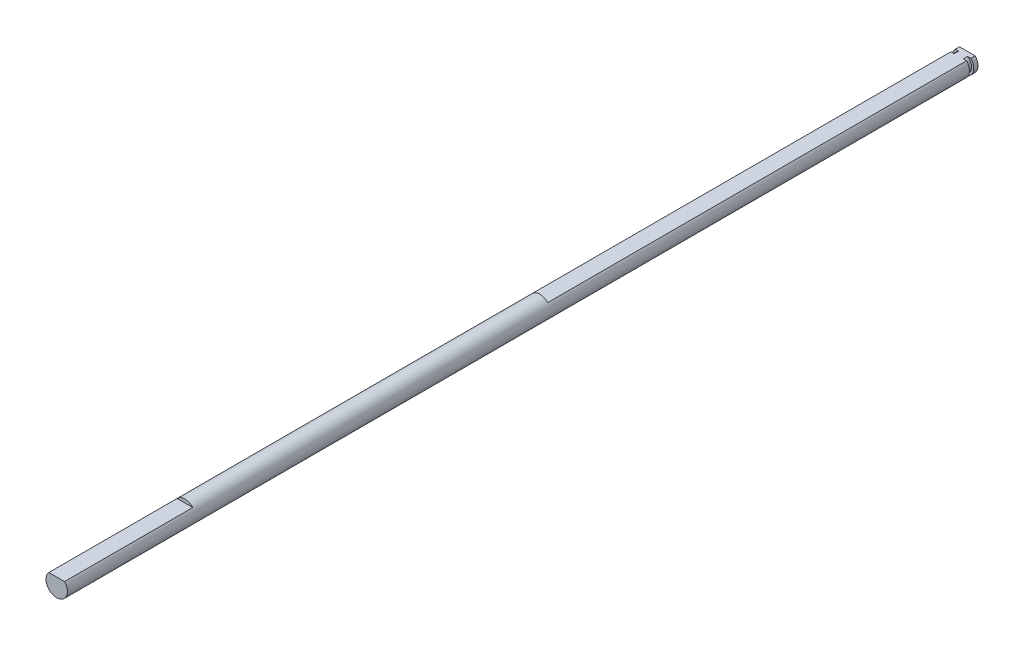
from build123d import *

# Parameters (mm, degrees)
SKETCH1_R           = 2.5
BOSS_EXTRUDE1_DEPTH = 213
CUT_EXTRUDE2_DEPTH  = 100
CUT_EXTRUDE3_START  = 1
SKETCH5_R           = 2.5
SKETCH5_R_2         = 2
CUT_EXTRUDE3_DEPTH  = 1
CUT_EXTRUDE4_START  = -30
CUT_EXTRUDE4_DEPTH  = 30


with BuildPart() as part:
    # Sketch1 → Boss-Extrude1 (new body)
    with BuildSketch(Plane.XY):
        Circle(SKETCH1_R)
    extrude(amount=BOSS_EXTRUDE1_DEPTH)

    # Sketch4 → Cut-Extrude2 (cut)
    with BuildSketch(Plane(origin=(0, 0, 0), x_dir=(-1, 0, 0), z_dir=(0, 0, -1))):
        with BuildLine():
            Line((-1.833030278, 1.7), (1.833030278, 1.7))
            ThreePointArc((1.833030278, 1.7), (0, 2.5), (-1.833030278, 1.7))
        make_face()
    extrude(amount=-CUT_EXTRUDE2_DEPTH, mode=Mode.SUBTRACT)

    # Sketch5 → Cut-Extrude3 (cut)
    with BuildSketch(Plane(origin=(0, 0, 2), x_dir=(-1, 0, 0), z_dir=(0, 0, -1)).offset(CUT_EXTRUDE3_START)):
        with Locations(Location((0, 0, 0), (0, 0, 42.843643044))):
            Circle(SKETCH5_R)
        Circle(SKETCH5_R_2, mode=Mode.SUBTRACT)
    extrude(amount=-CUT_EXTRUDE3_DEPTH, mode=Mode.SUBTRACT)

    # Sketch7 → Cut-Extrude4 (cut)
    with BuildSketch(Plane.XY.offset(213).offset(CUT_EXTRUDE4_START)):
        with BuildLine():
            Line((-1.835, 1.69787367), (1.835, 1.69787367))
            ThreePointArc((1.835, 1.69787367), (0, 2.5), (-1.835, 1.69787367))
        make_face()
    extrude(amount=CUT_EXTRUDE4_DEPTH, mode=Mode.SUBTRACT)


solid = part.part
